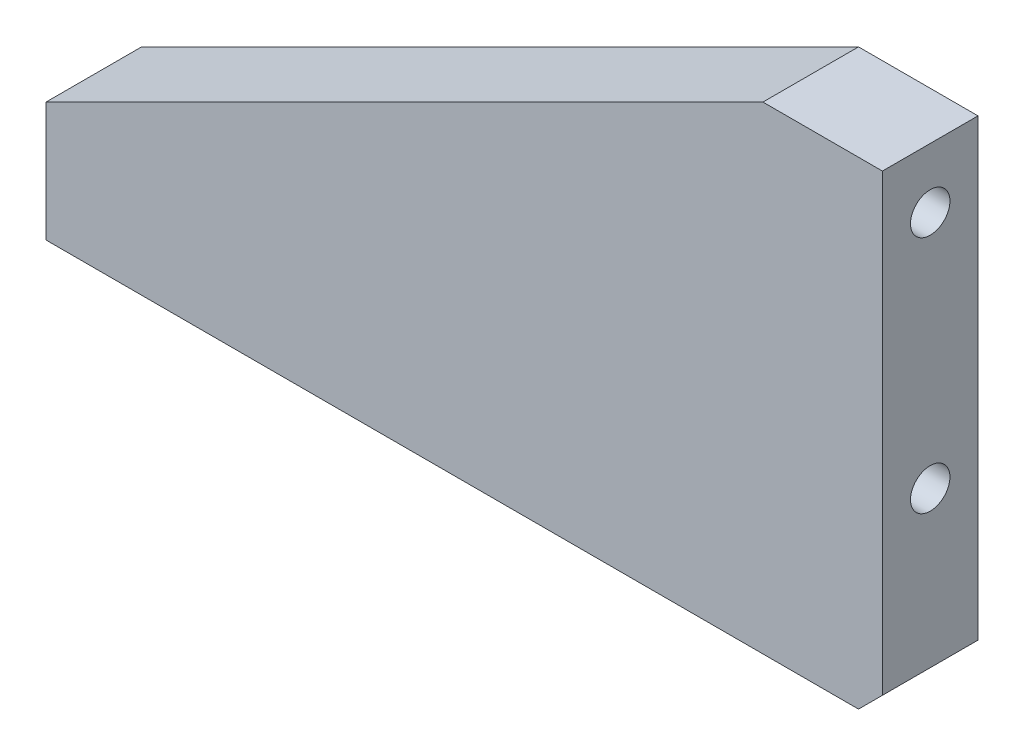
SolidWorks part; units mm, degrees
material "A6061"
ref_plane "前基準面" through (0, 0, 0) normal (0, 0, 1) x (1, 0, 0)
ref_plane "上基準面" through (0, 0, 0) normal (0, 1, 0) x (1, 0, 0)
ref_plane "右基準面" through (0, 0, 0) normal (1, 0, 0) x (0, 0, -1)
sketch "草图1" plane through (0, 0, 0) normal (0, 0, 1) x (1, 0, 0)
  line L0 (0, 0) -> (0, 40)
  line L1 (0, 40) -> (-10, 40)
  line L2 (-10, 40) -> (-70, 10)
  line L3 (-70, 10) -> (-70, 0)
  line L4 (-70, 0) -> (0, 0)
  dimension "D1" = 10
  dimension "D2" = 10
  dimension "D3" = 40
  dimension "D4" = 70
extrude "凸台-拉伸1" add sketch "草图1" along normal blind 8
sketch "草图2" plane through (0, 0, 0) normal (0, -1, 0) x (-1, 0, 0)
  line L0 (70, -4) -> (74.7899, -4) construction
  line L1 (70, -8) -> (70, 0) construction
  point P0 (15, -4)
  point P2 (65, -4)
  dimension "D1" = 5
  dimension "D2" = 50
hole_wizard "M4 螺纹孔2" positions "草图2" profile "草图3" tap size "M4" standard "GB"
sketch "草图3" plane through (-15, 0, 4) normal (1, 0, 0) x (0, 0, -1)
  line L0 (0, 0) -> (0, 11.0914)
  line L1 (0, 11.0914) -> (1.65, 10.1)
  line L2 (1.65, 10.1) -> (1.65, 0)
  line L5 (1.65, 0) -> (0, 0)
  line L10 (0, 11.0914) -> (-1.65, 10.1) construction
  line L11 (0, -6.35) -> (0, 107.95) construction
  dimension "螺纹孔钻头直径" = 3.3
  dimension "螺纹孔钻头深度" = 10.1
  dimension "导头角度" = 118
cosmetic thread "孔螺纹线1" parameters "D1"=8, "D2"=4
cosmetic thread "孔螺纹线2" parameters "D1"=8, "D2"=4
sketch "草图4" plane through (0, 0, 0) normal (1, 0, 0) x (0, 0, -1)
  line L0 (-8, 40) -> (0, 40) construction
  point P0 (-4, 35)
  point P2 (-4, 15)
  dimension "D1" = 5
  dimension "D2" = 20
hole_wizard "M4 螺纹孔1" positions "草图4" profile "草图5" tap size "M4" standard "GB"
sketch "草图5" plane through (0, 35, 4) normal (0, 1, 0) x (0, 0, -1)
  line L0 (0, 0) -> (0, 11.0914)
  line L1 (0, 11.0914) -> (1.65, 10.1)
  line L2 (1.65, 10.1) -> (1.65, 0)
  line L5 (1.65, 0) -> (0, 0)
  line L10 (0, 11.0914) -> (-1.65, 10.1) construction
  line L11 (0, -6.35) -> (0, 107.95) construction
  dimension "螺纹孔钻头直径" = 3.3
  dimension "螺纹孔钻头深度" = 10.1
  dimension "导头角度" = 118
cosmetic thread "孔螺纹线3" parameters "D1"=8, "D2"=4
cosmetic thread "孔螺纹线4" parameters "D1"=8, "D2"=4
chamfer "倒角1" distance 2 angle 45 1 edges at (0, 0, 4)
